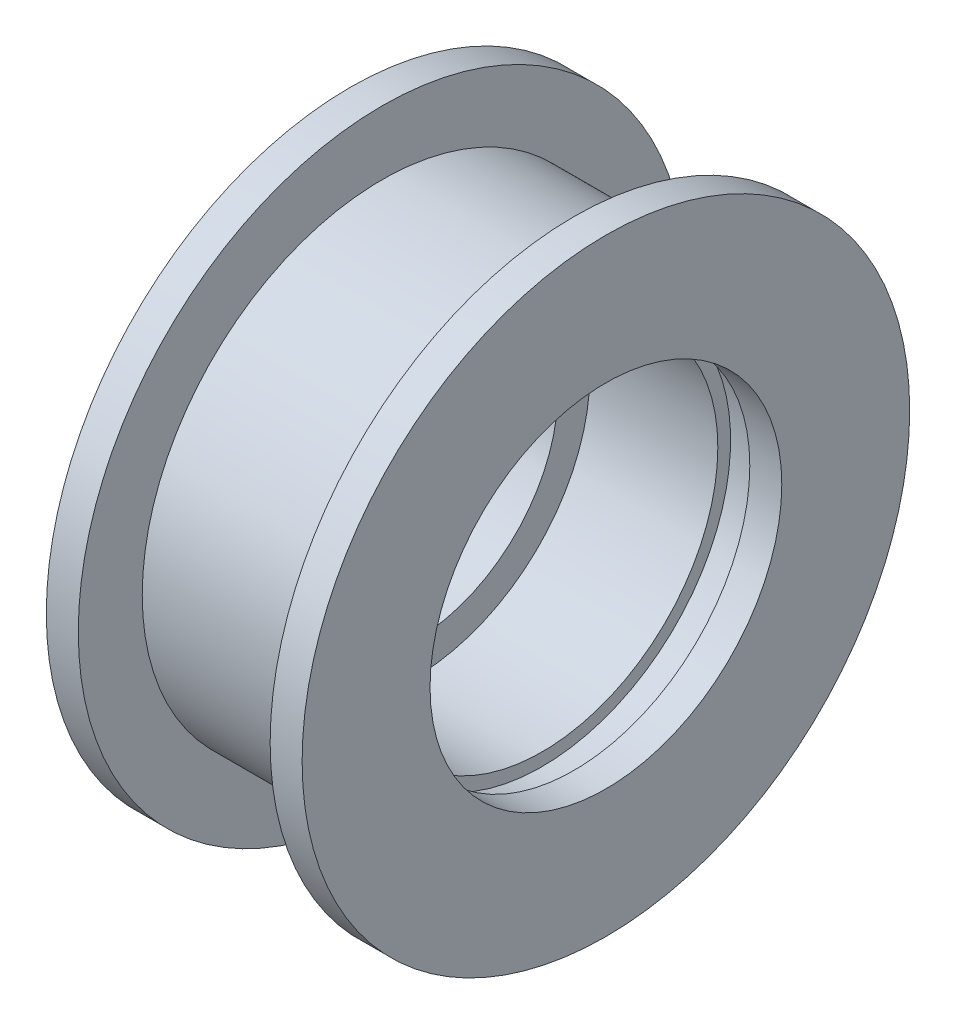
from build123d import *


with BuildPart() as part:
    # 草图1 → 旋转1 (revolve)
    with BuildSketch(Plane.XY, mode=Mode.PRIVATE) as revolve_1_sk:
        Polygon((-4, 4.5), (-2, 4.5), (-2, 5.5), (2, 5.5), (2, 5.9), (3, 5.9), (3, 5.5), (4, 5.5), (4, 9.5), (3, 9.5), (3, 7.5), (-3, 7.5), (-3, 9.5), (-4, 9.5), align=None)
    revolve(revolve_1_sk.sketch.rotate(Axis((4, 0, 0), (-1, 0, 0)), 270), axis=Axis((4, 0, 0), (-1, 0, 0)))


solid = part.part
